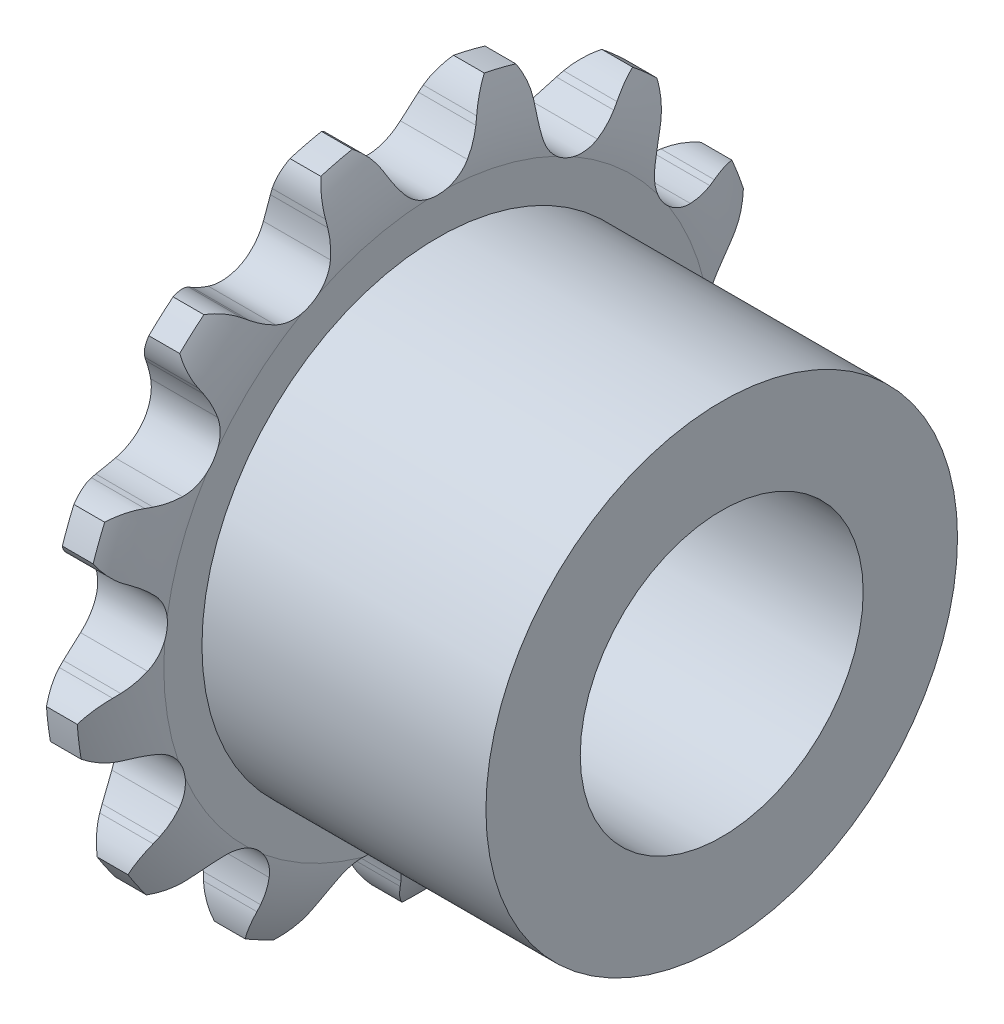
from build123d import *

# Parameters (mm, degrees)
EXTRUDECUTONE_DEPTH = 2.537198082
PATTERNONE_COUNT    = 13


with BuildPart() as part:
    # Sketch1 → Revolve 2 (revolve)
    with BuildSketch(Plane.XY, mode=Mode.PRIVATE) as revolve_2_sk:
        with BuildLine():
            Line((-1.4787, 6), (-1.4787, 9))
            Line((-1.4787, 9), (-1.4787, 11.616996164))
            ThreePointArc((-1.4787, 11.616996164), (-1.238582344, 13.107928471), (-0.6532, 14.5))
            Line((-0.6532, 14.5), (0.6532, 14.5))
            ThreePointArc((0.6532, 14.5), (1.238582344, 13.107928471), (1.4787, 11.616996164))
            Line((1.4787, 11.616996164), (1.4787, 10))
            Line((1.4787, 10), (13.5213, 10))
            Line((13.5213, 10), (13.5213, 6))
            Line((13.5213, 6), (-1.4787, 6))
        make_face()
    revolve(revolve_2_sk.sketch.rotate(Axis((-4, 0, 0), (1, 0, 0)), 90), axis=Axis((-4, 0, 0), (1, 0, 0)))

    # Sketch2 → ExtrudeCutOne (cut, symmetric)
    with BuildSketch(Plane(origin=(0, 0, 0), x_dir=(0, 0, -1), z_dir=(1, 0, 0))):
        with BuildLine():
            Line((1.877033772, 13.04944298), (1.99623343, 13.294673565))
            ThreePointArc((1.99623343, 13.294673565), (2.33688783, 13.81304378), (2.798488381, 14.227384256))
            ThreePointArc((2.798488381, 14.227384256), (0, 14.5), (-2.798488381, 14.227384256))
            ThreePointArc((-2.798488381, 14.227384256), (-2.33688783, 13.81304378), (-1.99623343, 13.294673565))
            Line((-1.99623343, 13.294673565), (-1.877033772, 13.04944298))
            ThreePointArc((-1.877033772, 13.04944298), (-1.622555123, 12.596822066), (-1.315936822, 12.177763249))
            ThreePointArc((-1.315936822, 12.177763249), (0, 11.558746164), (1.315936822, 12.177763249))
            ThreePointArc((1.315936822, 12.177763249), (1.622555123, 12.596822066), (1.877033772, 13.04944298))
        make_face()
    extrudecutone = extrude(amount=EXTRUDECUTONE_DEPTH, both=True, mode=Mode.SUBTRACT)

    # PatternOne: ExtrudeCutOne ×13 about axis
    patternone_axis = Axis((0, 0, 0), (1, 0, 0))
    for i in range(1, PATTERNONE_COUNT):
        add(extrudecutone.rotate(patternone_axis, i * 360 / PATTERNONE_COUNT), mode=Mode.SUBTRACT)


solid = part.part
